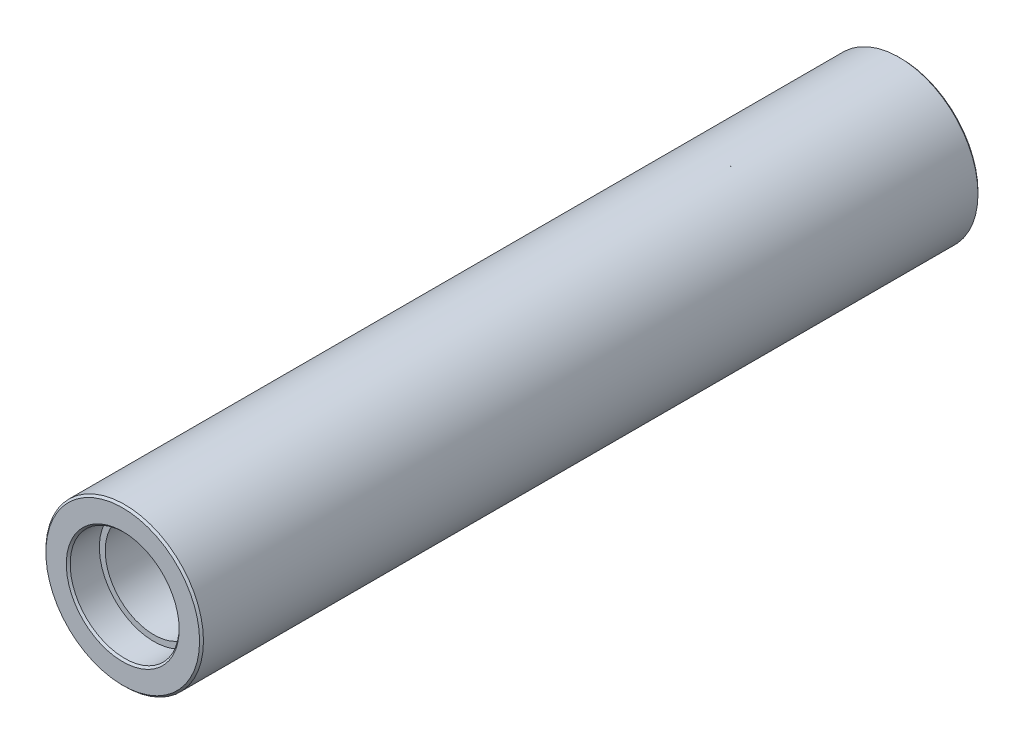
SolidWorks part; units mm, degrees
ref_plane "前视基准面" through (0, 0, 0) normal (0, 0, 1) x (1, 0, 0)
ref_plane "上视基准面" through (0, 0, 0) normal (0, 1, 0) x (1, 0, 0)
ref_plane "右视基准面" through (0, 0, 0) normal (1, 0, 0) x (0, 0, -1)
sketch "草图1" plane through (0, 0, 0) normal (0, 0, 1) x (1, 0, 0)
  circle A0 centre (0, 0) radius 20.25
  dimension "D1" = 40.5
extrude "凸台-拉伸1" add sketch "草图1" along normal mid plane 200
sketch "草图2" plane through (0, 0, 100) normal (0, 0, 1) x (1, 0, 0)
  circle A0 centre (0, 0) radius 14
  dimension "D1" = 28
extrude "切除-拉伸1" cut sketch "草图2" against normal blind 8
mirror "镜向1" about plane through (0, 0, 0) normal (0, 0, 1) of "切除-拉伸1"
sketch "草图3" plane through (0, 0, 92) normal (0, 0, 1) x (1, 0, 0)
  circle A0 centre (0, 0) radius 12.5
  dimension "D1" = 25
extrude "切除-拉伸2" cut sketch "草图3" against normal through all
chamfer "倒角1" distance 0.5 angle 45 4 edges at (14, 0, 100) (14, 0, -100) (20.25, 0, -100) (20.25, 0, 100)
